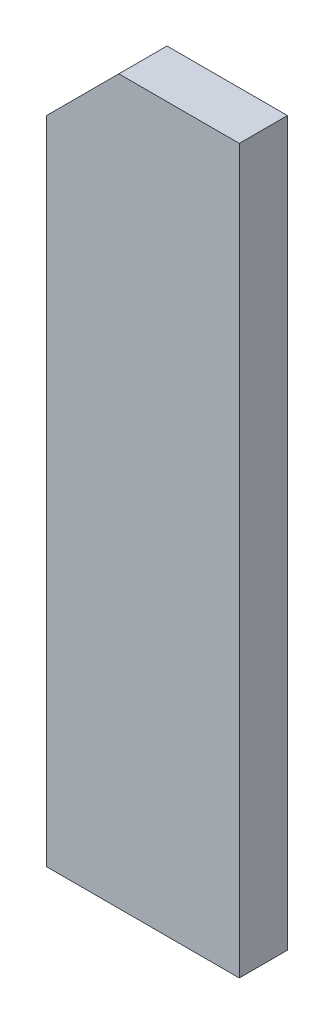
from build123d import *

# Parameters (mm, degrees)
BOSS_EXTRUDE1_DEPTH = 20


with BuildPart() as part:
    # Sketch1 → Boss-Extrude1 (new body)
    with BuildSketch(Plane.XY):
        Polygon((-50, 300), (-80, 270), (-80, 0), (0, 0), (0, 300), align=None)
    extrude(amount=BOSS_EXTRUDE1_DEPTH)


solid = part.part
